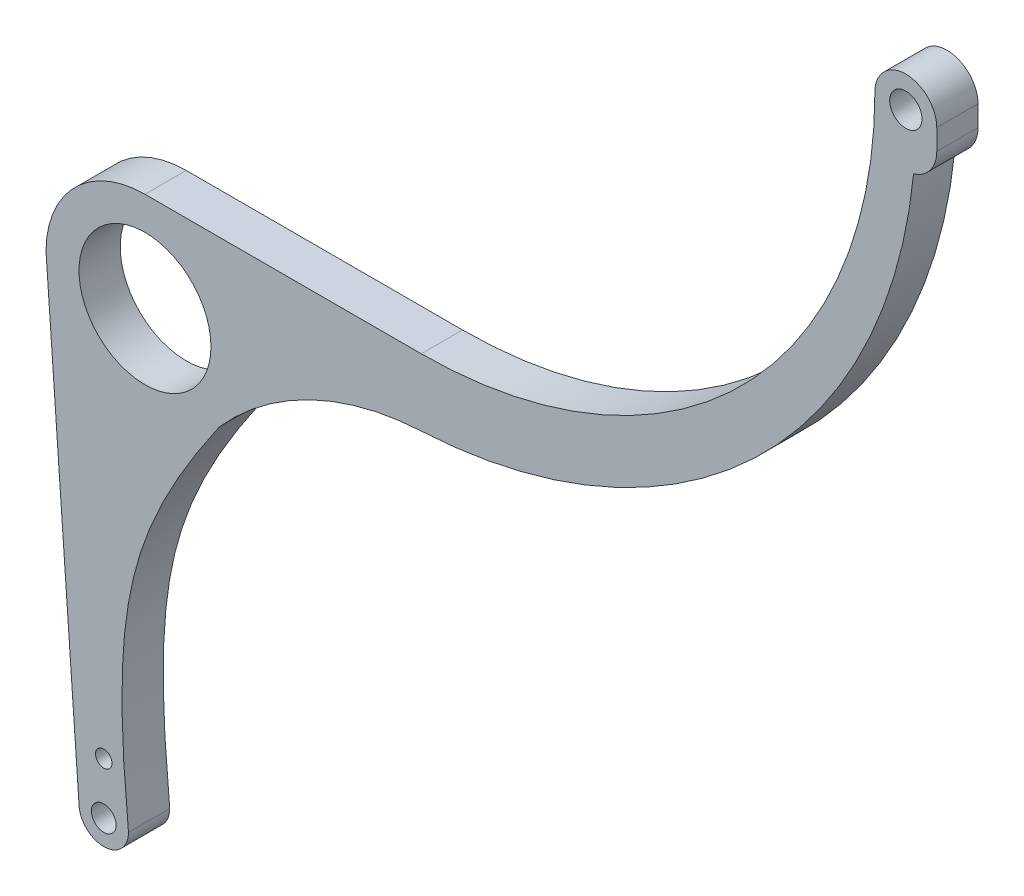
SolidWorks part; units mm, degrees
ref_plane "前视基准面" through (0, 0, 0) normal (0, 0, 1) x (1, 0, 0)
ref_plane "上视基准面" through (0, 0, 0) normal (0, 1, 0) x (1, 0, 0)
ref_plane "右视基准面" through (0, 0, 0) normal (1, 0, 0) x (0, 0, -1)
other "Configuration Table"
sketch "草图1" plane through (0, 0, 0) normal (0, 0, 1) x (1, 0, 0)
  line L0 (-60.8711, 0) -> (72.3657, 0) construction
  line L1 (-84.052, 112) -> (106.5467, 112) construction
  line L2 (0, 12.5) -> (0, -18.0859) construction
  line L3 (0, -18.0859) -> (10, -18.0859) construction
  line L4 (10, -18.0859) -> (10, 407.7959) construction
  line L5 (-9, 59.8208) -> (-9, -18.0859) construction
  line L6 (-14, 112) -> (-6, 0)
  line L7 (-176.4012, 246) -> (270.3663, 246) construction
  line L8 (77, 485.9134) -> (77, 110.3328) construction
  line L9 (10, 136) -> (77, 136)
  line L10 (187, 246) -> (194.5, 246) construction
  line L11 (202, 246) -> (202, 241)
  line L12 (202, 241) -> (194.1788, 241) construction
  line L13 (70.6056, 267.7759) -> (70.6056, 254.1409) construction
  line L14 (4.2515, 49.8248) -> (157.9856, 49.8248) construction
  line L15 (80.543, 130.5208) -> (80.543, 47.5555) construction
  line L16 (4.7446, 96.1309) -> (49.2871, 96.1309) construction
  line L17 (-29.78, 356) -> (265.8488, 356) construction
  circle A0 centre (0, 0) radius 3
  arc A1 (-6, 0) -> (6, 0) centre (0, 0) ccw
  circle A2 centre (10, 112) radius 16
  arc A3 (10, 136) -> (-14, 112) centre (10, 112) ccw
  circle A4 centre (77, 246) radius 115 construction
  arc A5 (77, 136) -> (187, 246) centre (77, 246) ccw
  arc A6 (202, 246) -> (187, 246) centre (194.5, 246) ccw
  arc A9 (196.3799, 233.4949) -> (202, 241) centre (194.1788, 241) ccw
  arc A10 (77, 119.7674) -> (28.0048, 96.1309) centre (80.543, 49.8248) ccw
  arc A11 (77, 119.7674) -> (196.3799, 233.4949) centre (70.6056, 246) ccw
  circle A12 centre (194.5, 246) radius 3.919
  circle A13 centre (0, 12.5) radius 2
  spline S0 degree 3 poles (6, 0) (1.5887, 45.6809) (5.6041, 63.6432) (28.0048, 96.1309) knots 0 0 0 0 0.788155 0.788155 0.788155 0.788155
  dimension "D1" = 6
  dimension "D2" = 12
  dimension "D5" = 19
  dimension "D6" = 134
  dimension "D8" = 230
  dimension "D9" = 6.3944
  dimension "D10" = 62.1752
  dimension "D12" = 15.8691
  dimension "D14" = 24
  dimension "D15" = 4
  dimension "D16" = 7.838
  dimension "D17" = 7.5
  dimension "D18" = 220
  dimension "D3" = 112
  dimension "D4" = 9
  dimension "D7" = 67
  dimension "D11" = 70.543
  dimension "D13" = 12.5
extrude "凸台-拉伸1" add sketch "草图1" along normal blind 10
